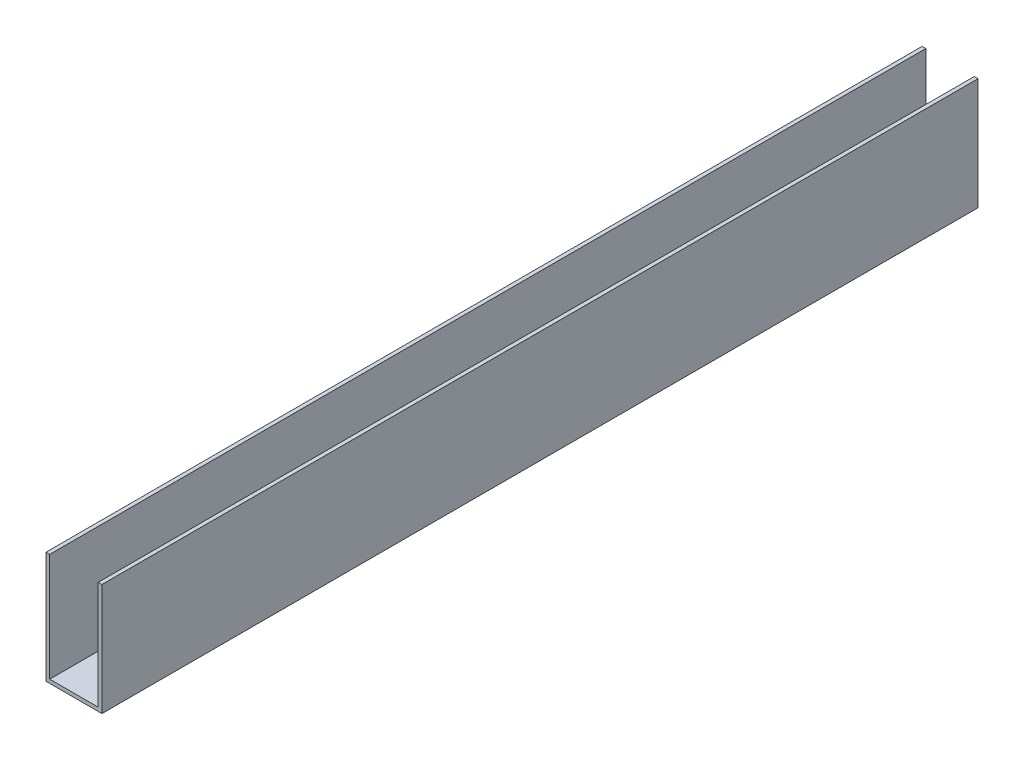
SolidWorks part; units mm, degrees
material "标准件"
ref_plane "前视基准面" through (0, 0, 0) normal (0, 0, 1) x (1, 0, 0)
ref_plane "上视基准面" through (0, 0, 0) normal (0, 1, 0) x (1, 0, 0)
ref_plane "右视基准面" through (0, 0, 0) normal (1, 0, 0) x (0, 0, -1)
sketch "草图1" plane through (0, 0, 0) normal (0, 0, 1) x (1, 0, 0)
  line L0 (0, 0) -> (0, 33.955) construction
  line L2 (-15, -30) -> (15, -30)
  line L3 (-15, -30) -> (-15, 30)
  line L4 (-15, 30) -> (15, 30)
  line L5 (15, -30) -> (15, 30)
  line L6 (-15, -30) -> (15, 30) construction
  line L7 (-15, 30) -> (15, -30) construction
  dimension "D1" = 30
  dimension "D2" = 60
extrude "凸台-拉伸1" add sketch "草图1" along normal mid plane 470
shell "抽壳1" thickness 2
